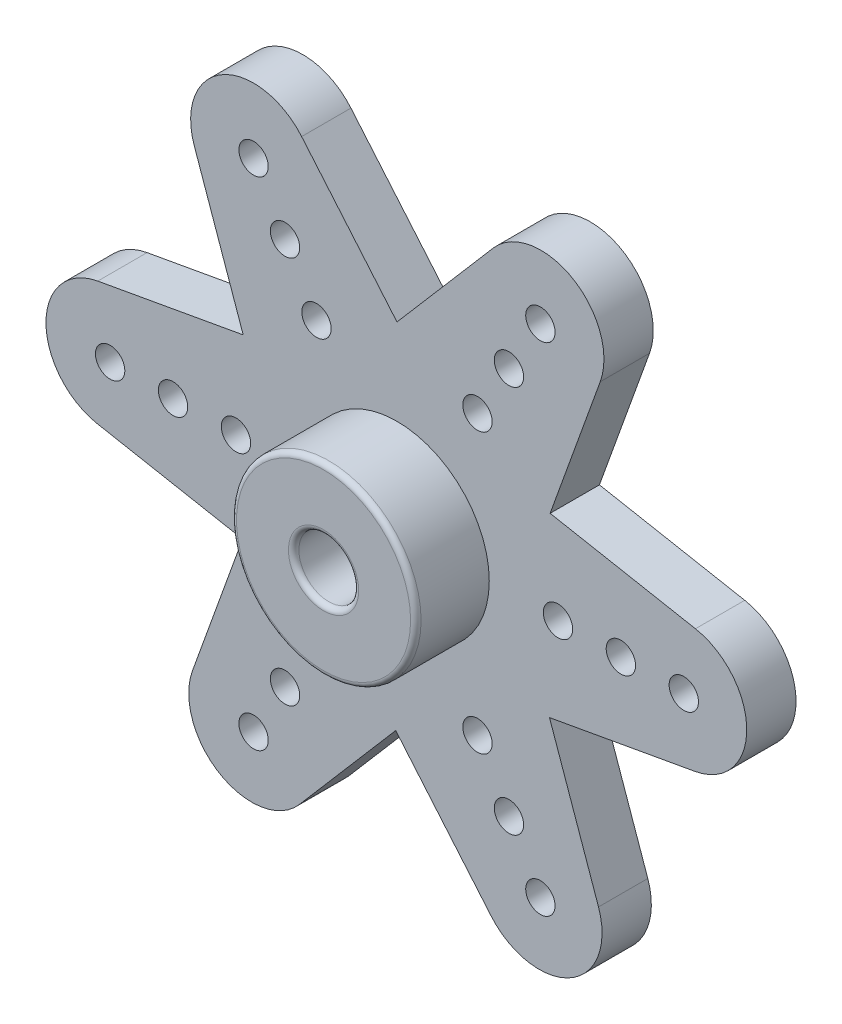
SolidWorks part; units mm, degrees
ref_plane "前视基准面" through (0, 0, 0) normal (0, 0, 1) x (1, 0, 0)
ref_plane "上视基准面" through (0, 0, 0) normal (0, 1, 0) x (1, 0, 0)
ref_plane "右视基准面" through (0, 0, 0) normal (1, 0, 0) x (0, 0, -1)
sketch "草图1" plane through (0, 0, 0) normal (0, 0, 1) x (1, 0, 0)
  line L0 (0, 0) -> (2.8267, 0) construction
  line L1 (0, 0) -> (0, -1.5782) construction
  line L2 (-4.545, 13.8823) -> (0, 8.5)
  line L3 (0, 8.5) -> (4.5913, 13.8487)
  line L4 (9.6899, 10.8775) -> (7.3013, 4.2502)
  line L5 (7.3013, 4.2502) -> (14.229, 2.9484)
  line L6 (14.2052, -2.9528) -> (7.2715, -4.1978)
  line L7 (7.2715, -4.1978) -> (9.608, -10.8483)
  line L8 (4.4855, -13.7782) -> (-0.0596, -8.396)
  line L9 (-0.0596, -8.396) -> (-4.6509, -13.7447)
  line L10 (-9.7495, -10.7734) -> (-7.3608, -4.1462)
  line L11 (-7.3608, -4.1462) -> (-14.2886, -2.8444)
  line L12 (-14.2648, 3.0568) -> (-7.3311, 4.3018)
  line L13 (-7.3311, 4.3018) -> (-9.6675, 10.9523)
  circle A8 centre (0, 0) radius 13.675 construction
  circle A9 centre (0, 0) radius 8.5 construction
  arc A10 (14.2052, -2.9528) -> (14.229, 2.9484) centre (13.675, 0) ccw
  arc A11 (4.4855, -13.7782) -> (9.608, -10.8483) centre (6.7776, -11.8427) ccw
  arc A12 (-9.7495, -10.7734) -> (-4.6509, -13.7447) centre (-6.9272, -11.7907) ccw
  arc A13 (-14.2648, 3.0568) -> (-14.2886, -2.8444) centre (-13.7346, 0.104) ccw
  arc A14 (-4.545, 13.8823) -> (-9.6675, 10.9523) centre (-6.8371, 11.9467) ccw
  arc A15 (9.6899, 10.8775) -> (4.5913, 13.8487) centre (6.8677, 11.8947) ccw
  circle A16 centre (13.675, 0) radius 0.7
  circle A17 centre (10.675, 0) radius 0.7
  circle A18 centre (7.675, 0) radius 0.7
  circle A19 centre (3.8375, -6.6467) radius 0.7
  circle A20 centre (5.3375, -9.2448) radius 0.7
  circle A21 centre (6.8375, -11.8429) radius 0.7
  circle A22 centre (-3.8375, -6.6467) radius 0.7
  circle A23 centre (-5.3375, -9.2448) radius 0.7
  circle A24 centre (-6.8375, -11.8429) radius 0.7
  circle A25 centre (-7.675, 0) radius 0.7
  circle A26 centre (-10.675, 0) radius 0.7
  circle A27 centre (-13.675, 0) radius 0.7
  circle A28 centre (-3.8375, 6.6467) radius 0.7
  circle A29 centre (-5.3375, 9.2448) radius 0.7
  circle A30 centre (-6.8375, 11.8429) radius 0.7
  circle A31 centre (3.8375, 6.6467) radius 0.7
  circle A32 centre (5.3375, 9.2448) radius 0.7
  circle A33 centre (6.8375, 11.8429) radius 0.7
  dimension "D1" = 27.35
  dimension "D2" = 17
  dimension "D5" = 6
  dimension "D6" = 1.4
  dimension "D7" = 3
  dimension "D8" = 3
  dimension "D3" = 6
  dimension "D4" = 6
extrude "凸台-拉伸1" add sketch "草图1" along normal blind 2.35
sketch "草图2" plane through (0, 0, 2.35) normal (0, 0, 1) x (1, 0, 0)
  circle A0 centre (0, 0) radius 4.4
  dimension "D1" = 8.8
extrude "凸台-拉伸2" add sketch "草图2" along normal blind 3.5
sketch "草图3" plane through (0, 0, 5.85) normal (0, 0, 1) x (1, 0, 0)
  circle A0 centre (0, 0) radius 1.425
  dimension "D1" = 2.85
extrude "切除-拉伸1" cut sketch "草图3" against normal through all
fillet "圆角1" radius 0.25 2 edges at (4.4, 0, 5.85) (1.425, 0, 5.85)
sketch "草图4" plane through (0, 0, 0) normal (0, 0, -1) x (-1, 0, 0)
  circle A0 centre (0, 0) radius 4.25
  circle A1 centre (0, 0) radius 3.5
  circle A2 centre (0, 0) radius 3
  dimension "D1" = 8.5
  dimension "D2" = 7
  dimension "D3" = 6
extrude "切除-拉伸2" cut sketch "草图4" against normal blind 1 contours A1 | A0
sketch "草图5" plane through (0, 0, 0) normal (0, 0, -1) x (-1, 0, 0)
  circle A0 centre (0, 0) radius 3
  dimension "D1" = 6
extrude "切除-拉伸3" cut sketch "草图5" against normal blind 1
